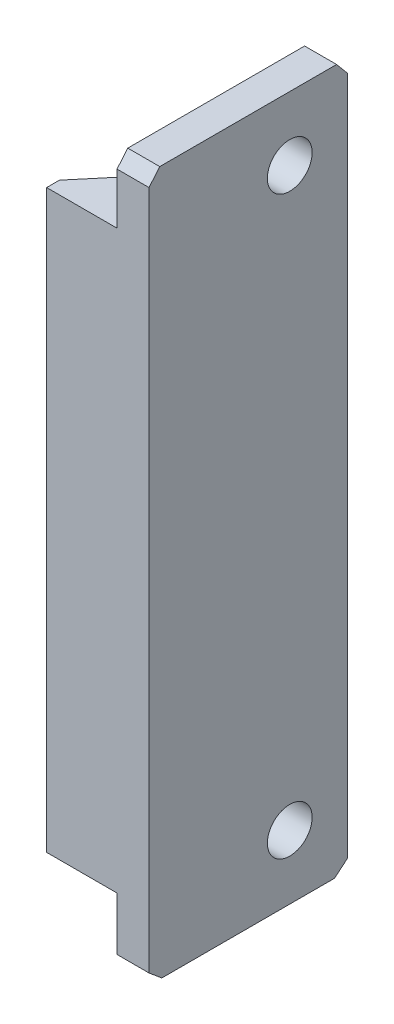
SolidWorks part; units mm, degrees
material "AISI 304"
ref_plane "Front Plane" through (0, 0, 0) normal (0, 0, 1) x (1, 0, 0)
ref_plane "Top Plane" through (0, 0, 0) normal (0, 1, 0) x (1, 0, 0)
ref_plane "Right Plane" through (0, 0, 0) normal (1, 0, 0) x (0, 0, -1)
sketch "Sketch1" plane through (0, 0, 0) normal (0, 1, 0) x (1, 0, 0)
  line L1 (0, 0) -> (8, 0)
  line L2 (0, 0) -> (0, 15.5)
  line L3 (0, 15.5) -> (8, 15.5)
  line L4 (8, 0) -> (8, 15.5)
  dimension "D1" = 8
  dimension "D2" = 15.5
extrude "Boss-Extrude1" add sketch "Sketch1" along normal blind 55
sketch "Sketch2" plane through (0, 55, 0) normal (0, 1, 0) x (1, 0, 0)
  line L0 (8, 0) -> (8, 15.5) construction
  line L1 (0, 15.5) -> (5.5, 15.5)
  line L2 (0, 15.5) -> (0, 4)
  line L3 (0, 4) -> (5.5, 4)
  line L4 (5.5, 15.5) -> (5.5, 4)
  line L5 (0, 0) -> (8, 0) construction
  dimension "D1" = 2.5
  dimension "D2" = 4
extrude "Cut-Extrude1" cut sketch "Sketch2" against normal through all
chamfer "Chamfer1" distance 3 angle 40 1 edges at (0, 27.5, -4)
sketch "Sketch3" plane through (8, 0, 0) normal (1, 0, 0) x (0, 0, -1)
  line L0 (0, 27.5) -> (50000, 27.5) construction
  line L1 (0, 55) -> (0, 0) construction
  circle A0 centre (11, 50) radius 1.75
  circle A1 centre (11, 5) radius 1.75
  point P4 (0, 27.5)
  dimension "D1" = 45
  dimension "D2" = 11
  dimension "D3" = 3.5
extrude "Cut-Extrude2" cut sketch "Sketch3" against normal blind 48
sketch "Sketch4" plane through (0, 0, -4) normal (0, 0, -1) x (-1, 0, 0)
  line L0 (-8, 27.5) -> (49992, 27.5) construction
  line L1 (-8, 55) -> (-8, 0) construction
  line L2 (-5.5, 0) -> (-5.5, 55) construction
  line L3 (0, 55) -> (-5.5, 55)
  line L4 (0, 55) -> (0, 50)
  line L5 (0, 50) -> (-5.5, 50)
  line L6 (-5.5, 55) -> (-5.5, 50)
  line L7 (-5.5, 0) -> (-5.5, 5)
  line L8 (0, 5) -> (-5.5, 5)
  line L9 (0, 0) -> (0, 5)
  line L10 (0, 0) -> (-5.5, 0)
  point P4 (-8, 27.5)
  dimension "D1" = 45
extrude "Cut-Extrude3" cut sketch "Sketch4" against normal through all
chamfer "Chamfer2" distance 1 angle 40 4 edges at (6.75, 0, -15.5) (6.75, 55, -15.5) (6.75, 0, 0) (6.75, 55, 0)
